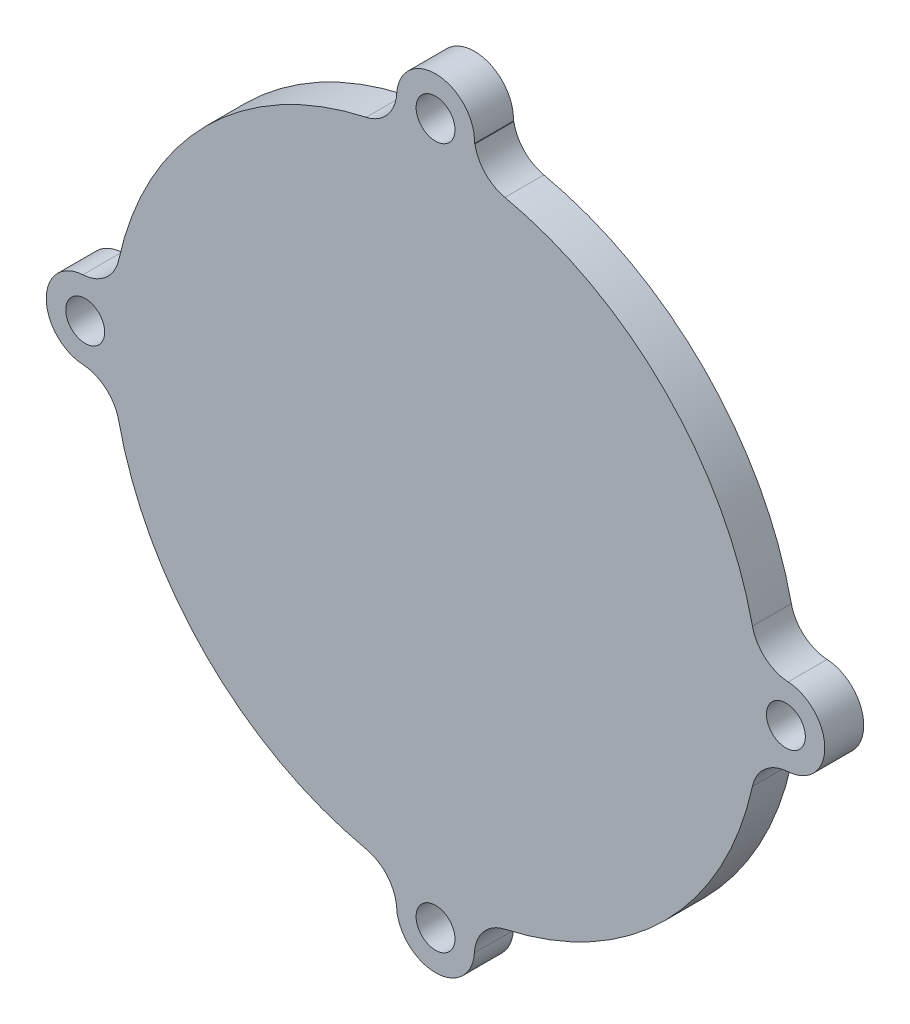
from build123d import *

# Parameters (mm, degrees)
SKETCH_1_R      = 1.5
EXTRUDE_1_DEPTH = 3


with BuildPart() as part:
    # 草图1 → 凸台-拉伸1 (new body)
    with BuildSketch(Plane.XY):
        with BuildLine():
            ThreePointArc((-3.035621948, 26.828809131), (-3.826001677, 25.273746937), (-5.347923635, 24.421296296))
            ThreePointArc((-5.347923635, 24.421296296), (-17.67766953, 17.67766953), (-24.421296296, 5.347923635))
            ThreePointArc((-24.421296296, 5.347923635), (-25.403311193, 3.708624428), (-27.175925926, 2.994837236))
            ThreePointArc((-27.175925926, 2.994837236), (-30, 0), (-27.175925926, -2.994837236))
            ThreePointArc((-27.175925926, -2.994837236), (-25.403311193, -3.708624428), (-24.421296296, -5.347923635))
            ThreePointArc((-24.421296296, -5.347923635), (-17.67766953, -17.67766953), (-5.347923635, -24.421296296))
            ThreePointArc((-5.347923635, -24.421296296), (-3.708624428, -25.403311193), (-2.994837236, -27.175925926))
            ThreePointArc((-2.994837236, -27.175925926), (0, -30), (2.994837236, -27.175925926))
            ThreePointArc((2.994837236, -27.175925926), (3.708624428, -25.403311193), (5.347923635, -24.421296296))
            ThreePointArc((5.347923635, -24.421296296), (17.67766953, -17.67766953), (24.421296296, -5.347923635))
            ThreePointArc((24.421296296, -5.347923635), (25.403311193, -3.708624428), (27.175925926, -2.994837236))
            ThreePointArc((27.175925926, -2.994837236), (30, 0), (27.175925926, 2.994837236))
            ThreePointArc((27.175925926, 2.994837236), (25.403311193, 3.708624428), (24.421296296, 5.347923635))
            ThreePointArc((24.421296296, 5.347923635), (17.67766953, 17.67766953), (5.347923635, 24.421296296))
            ThreePointArc((5.347923635, 24.421296296), (3.826001677, 25.273746937), (3.035621948, 26.828809131))
            ThreePointArc((3.035621948, 26.828809131), (3.015495219, 26.831078782), (2.995366793, 26.833333333))
            ThreePointArc((2.995366793, 26.833333333), (2.999996416, 27.004637195), (2.994837236, 27.175925926))
            ThreePointArc((2.994837236, 27.175925926), (0, 30), (-2.994837236, 27.175925926))
            ThreePointArc((-2.994837236, 27.175925926), (-2.999996416, 27.004637195), (-2.995366793, 26.833333333))
            ThreePointArc((-2.995366793, 26.833333333), (-3.015495219, 26.831078782), (-3.035621948, 26.828809131))
        make_face()
        with Locations((-27, 0)):
            Circle(SKETCH_1_R, mode=Mode.SUBTRACT)
        with Locations((0, -27)):
            Circle(SKETCH_1_R, mode=Mode.SUBTRACT)
        with Locations((27, 0)):
            Circle(SKETCH_1_R, mode=Mode.SUBTRACT)
        with Locations((0, 27)):
            Circle(SKETCH_1_R, mode=Mode.SUBTRACT)
    extrude(amount=EXTRUDE_1_DEPTH)


solid = part.part
